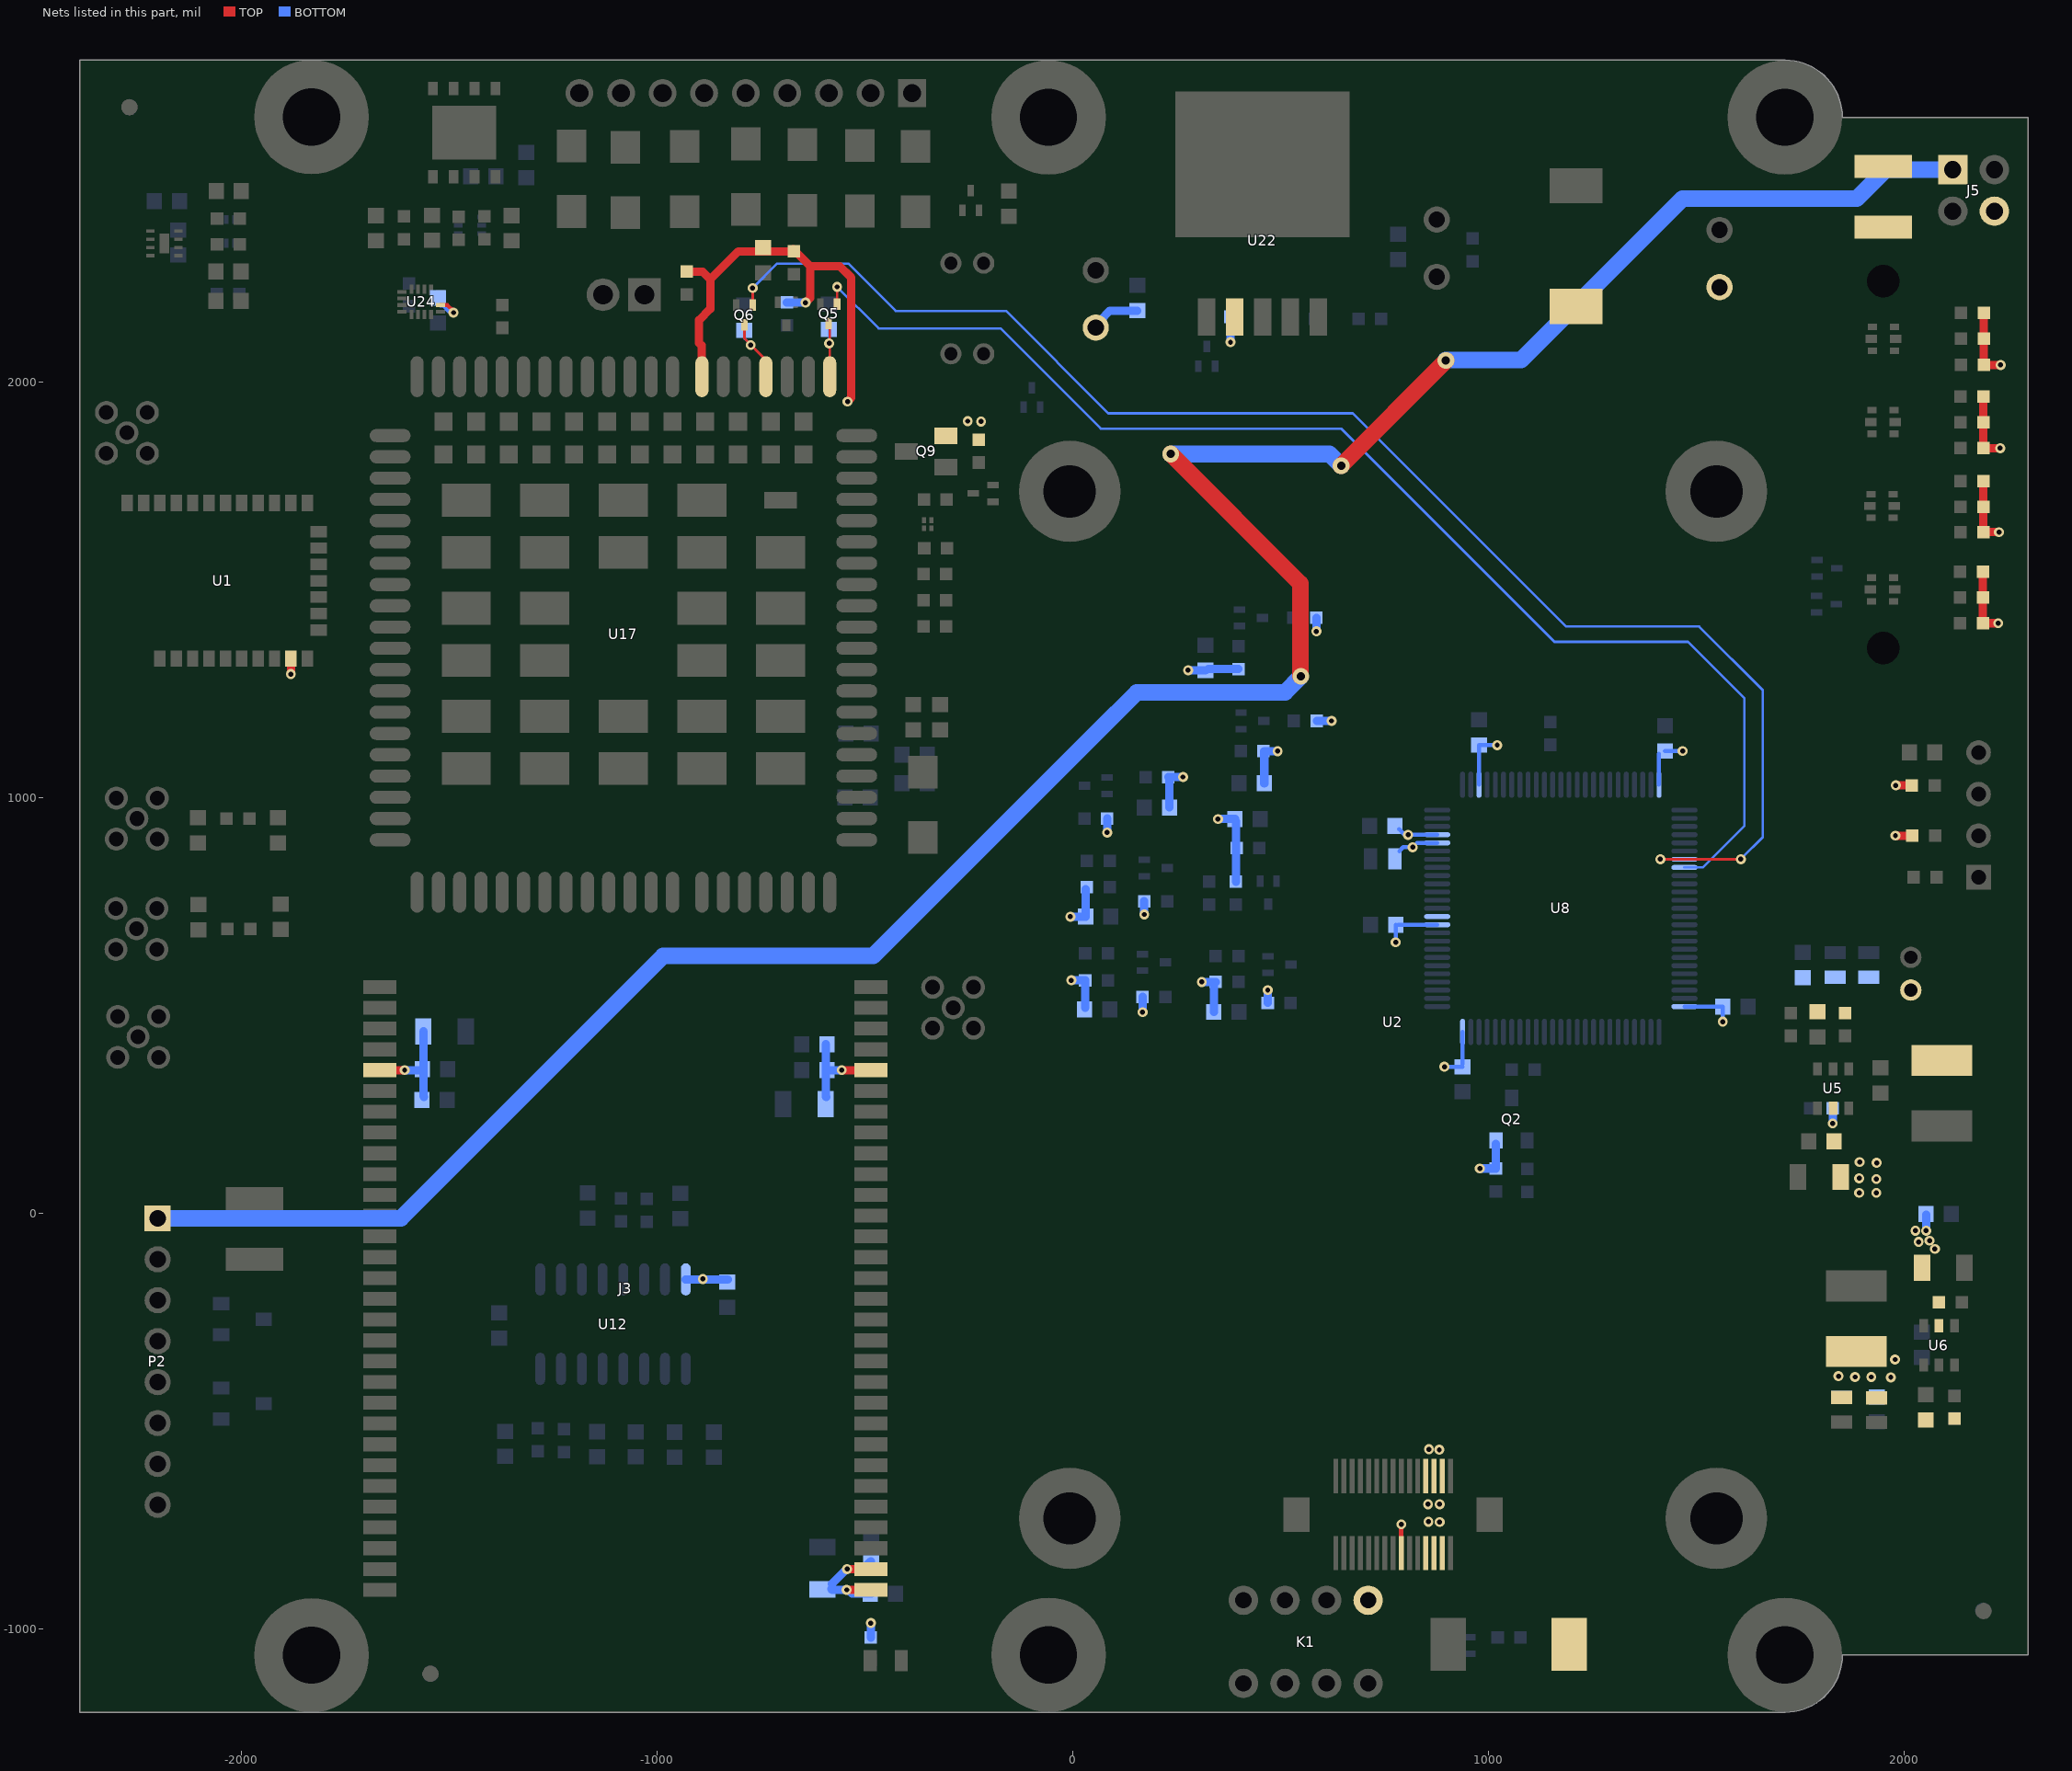
[diagram p0: the nets of this part, all layers, seen from the top]
# Altium PCB MISC84456.PcbDoc (part 5 of 5)
Units mil, origin at the board's own origin, x right, y up, seen from the top; angles counter-clockwise.
Board outline 4685.04 x 3973.82 mil, 4 copper layers (TOP, GND, POWER, BOTTOM), stack 38.4 mil thick; 219 components, 175 nets, 938 pads, 792 vias.

## Via types
v1: diameter 24, hole 12, TOP to BOTTOM, 400 vias
v2: diameter 24, hole 12, TOP to BOTTOM, tented both sides, 388 vias
v3: diameter 40, hole 20, TOP to BOTTOM, 4 vias

## Nets (pads, with @x,y where several pads share a name; then routed paths per layer and width w, separated by ;. In a path a pad name is that pad's centre, name@x,y a point inside that pad or via, vN(x,y) a via of type N, cw(c..) or ccw(c..) an arc to the next point about the centre after c; other vN are vias at no path point) (continued)
VDD_3V3: C2.1 C3.1 C11.1 C20.2 C21.2 C22.2 C38.2 C39.1 C40.1 C41.1 C42.1 C43.1 C53.1 C54.1 C55.2 C56.1 C88.1 J3.31 J3.32 J5.4 L4.2 Q2.2 R1.1 R2.1 R3.1 R17.2 R18.1 R25.2 R35.2 R38.2 R46.2 R49.2 R53.2 R55.2 R75.1 R76.1 R81.1 R82.1 R85.1 R86.1 R91.1 R92.1 R94.1 U1.9 U2.18 U2.23 U2.24 U2.25 U2.26 U2.27 U2.28 U8.11 U8.21 U8.22 U8.28 U8.50 U8.75 U8.100 U12.16 U24.14 | length 2443
  TOP w9: U24.14@-1520.59,2185.13 -1504.13,2185.13 v2@-1491,2172 ; v2@-1491.91,2171.09 -1488.81,2168 v2@-1486,2168
  TOP w11: U2.18@789.69,-816.52 v1(789.69,-747.31)
  TOP w20: v1(-1880.61,1297.61) U1.9@-1880.61,1334.99 ; v2(-544,-905) J3.31@-485.45,-905 ; v2(-543,-855) J3.32@-485.45,-855 ; v1(1978,909) R25.2@2018.5,909 ; v1(1979,1030) R35.2@2017.5,1030 ; R1.1@2188.5,1420 v1(2225,1420) ; R1.1@2188.5,1424.5 R2.1@2188.5,1482 R3.1@2188.5,1544 ; R85.1@2189.5,1639 v2(2227,1639) ; R85.1@2189.5,1645.5 R91.1@2189.5,1700 R94.1@2189.5,1762 ; R82.1@2189.5,1841 v2(2230,1841) ; R82.1@2189.5,1845.5 R86.1@2189.5,1903 R92.1@2189.5,1965 ; R75.1@2190.5,2040.5 R75.1@2190.5,2041 ; R81.1@2190.5,2166 R76.1@2190.5,2104 R75.1@2190.5,2041 ; v2(2231,2041) R75.1@2190.5,2041
  BOTTOM w10: C38.2@-1521,2184.5 -1514.5,2184.5 -1500,2170 v2@-1495,2170 ; v2@-1495,2169 -1489,2169 -1491,2167 v2(-1489.71,2167) ; v1(776.32,652.69) C54.1@776.32,695 ; C54.1@782.25,694.75 U8.11@876.11,694.75 ; C56.1@784,925 797.71,911.29 v1@806,911.29 ; C55.2@785,872 794.5,881.5 v1@817.5,881.5 ; v1(806,911) v1@806,911.29 ; v1(817,881) v1@817.5,881.5 ; U8.21@876,891 827,891 v1@817.5,881.5 ; U8.21@876,891.6 U8.21@876.11,891.6 ; U8.22@876.11,911.29 v1@806,911.29 ; v1(893.32,353.32) C11.1@937,353.32 ; C11.1@937.13,359.87 U8.100@937.13,436.88 ; U8.28@976.5,1031.36 C2.1@976.5,1124.5 ; C2.1@977,1126.69 v1(1020.32,1126.69) ; U8.50@1409.57,1031.36 C3.1@1409.57,1105.43 ; C3.1@1424,1112.69 v1(1466.32,1112.69) ; U8.75@1470.59,497.9 C53.1@1561.1,497.9 ; v1(1562.69,461.69) C53.1@1562.69,498
  BOTTOM w20: v2(-1489.71,2167) v2@-1489.6,2167 ; U12.16@-931,-158.2 v2@-891,-158.2 ; v2(-890,-157.2) v2@-891,-158.2 ; C88.1@-830.2,-158.2 v2@-891,-158.2 ; C22.2@-581,-903 -579,-905 -540,-905 -531,-914 C21.2@-484.5,-914 ; C22.2@-580,-891 -544,-855 v2(-543,-855) -505,-855 C20.2@-486,-836 ; R18.1@-486,-1019.5 v2(-486,-985) ; v1(167.5,484.5) R55.2@167.5,521 ; v1(171.5,719.5) R46.2@171.5,751 ; R53.2@468.5,507 v1(468.5,537.5) ; R49.2@586.5,1185 v1(622,1185) ; v1(978.5,108.5) R38.2@1017,108.5 Q2.2@1017,168
  other v1: 882,-742 855,-741 854,-699 882,-699 881,-568 856,-567 1967,-394 1881,-393 1920,-393 1841,-391 1977,-351
VDD_5V: C5.2 C6.1 C7.1 C8.2 C9.2 C10.2 C25.1 C26.1 C27.1 C28.1 C29.1 C91.1 C101.1 J3.5 J3.56 L3.2 Q9.2 R11.2 R29.1 R65.2 U22.2 | length 652.7
  TOP w20: J3.5@-1666.55,345 v2(-1607,345) ; v2(-556,345) J3.56@-485.45,345
  BOTTOM w20: v2@-1603,345 C9.2@-1562.5,345 ; C10.2@-1562.16,438 -1562.16,282.16 C8.2@-1561,281 ; C7.1@-594.5,407 -594.5,281.5 C5.2@-593,280 ; C6.1@-592,345 v2(-556,345) ; C91.1@65,2148 88.69,2171.69 C101.1@155,2171.69 ; R65.2@378.5,2157 378.5,2099.5 379,2099 v2(379,2096)
  other v2: -221,1905 -253,1906
VDD_12V: C4.1 C30.2 C31.2 C44.2 C46.2 D1.2 D3.2 K1.1 R10.1 R12.2 R19.2 U5.5 U6.5 | length 68.5
  BOTTOM w20: v1@1827.5,222.5 R12.2@1827.5,253 ; v2(2052,-41) C46.2@2052,-3
  other v1: 1827,217
  other v2: 2073,-85 2034,-68 2060,-65 2026,-41 1891,50 1932,50 1932,83 1891,85 1933,122 1892,124
VDD_EXT: C57.1 C58.2 C59.1 C60.1 C61.2 C62.2 C63.2 C64.2 R30.1 R31.1 R39.2 R40.2 R41.1 R43.2 R44.1 R45.1 R48.1 R51.1 R54.1 R56.1 R77.1 U17.7 | length 1990.2
  TOP w20: R77.1@-922,2265 -890,2265 -872,2247 ; U17.7@-893,2046 -893,2088 -899,2094 -899,2149 -872,2176 -872,2247 ; R31.1@-672.5,2319.5 -632,2279 ; R31.1@-671,2314.5 -804.5,2314.5 -872,2247 ; v2(-643,2191) -632,2202 -632,2279 ; v2(-542,1953) -533,1962 -533,2251 -561,2279 -632,2279
  BOTTOM w20: R30.1@-688,2191.5 v2@-643.5,2191.5 ; v1(-6,714) C61.2@30.69,714 R48.1@30.69,780.69 ; v1(-4,561) R56.1@29.5,561 C64.2@29.5,495.5 ; v1(82.5,916.5) R45.1@82.5,950 ; R43.2@229.5,1050 v1(265,1050) ; C60.1@232.32,977 R43.2@232.32,1048.69 ; v1(277,1307) C59.1@318.69,1307 ; v1(310,557) R54.1@343.5,557 ; C59.1@325.5,1309.5 R40.2@398,1309.5 ; C63.2@338.69,485 R54.1@338.69,549.69 ; v1(349,949) C57.1@389.69,949 ; R41.1@392,798.5 C57.1@392,943 ; C62.2@460.32,1035 460.32,1112.32 v1(492.32,1112.32) ; v1(585.5,1400.5) R44.1@585.5,1433
VDD_IN: J5.1 P2.1 R10.2 | length 6252
  TOP w40: v3(235,1827) 547,1515 v3@547,1293 ; v3(645,1799) v3@898,2052
  BOTTOM w40: P2.1@-2201,-11.51 -1616.51,-11.51 -985,620 -480,620 24,1124 ; 104,1204 24,1124 ; v3(235,1827) 617,1827 v3(645,1799) ; v3@547,1291 510,1254 154,1254 24,1124 ; v3@897,2053 1078,2053 1466,2441 1885,2441 1955,2511 J5.1@2116,2511
  other v3: 548,1292 897,2052
W_DISABLE_MCU: Q6.1 U8.57 | length 3759.8
  TOP w6: Q6.1@-770.12,2184.87 v2(-770.12,2226.12) ; v1(1412.77,852.23) v1(1606.23,852.23)
  BOTTOM w6: v2(-770.12,2226.12) -711.25,2285 -540,2285 -426,2171 -366,2171 ; -202,2171 -366,2171 ; v1(1412.77,852.23) U8.57@1470.59,852.23 ; v1@1609,855 1659,905 1659,1259 1506,1412 1186,1412 673,1925 85,1925 -161,2171 -366,2171
W_DISABLE_MODULE: C48.1 Q6.3 U17.4 | length 207
  TOP w6: Q6.3@-790,2141 -790,2105 -738.48,2053.48 U17.4@-738.48,2013.08
  BOTTOM w6: C48.1@-790,2120 C48.1@-790,2124.69 C48.1@-790,2135 ; C48.1@-789,2120 -789,2103.66 v2@-770.34,2085
  other v2: -775,2089
WAKEUP_IN_MCU: Q5.1 U8.58 | length 3247.2
  TOP w6: Q5.1@-567.12,2187.87 v2(-567.12,2228.88)
  BOTTOM w6: v2(-567.12,2228.88) -467.25,2129 -324,2129 ; -202,2129 -324,2129 ; U8.58@1470.59,832.55 1514.55,832.55 1615,933 1615,1239 1479,1375 1158,1375 645,1888 67,1888 -174,2129 -324,2129
WAKEUP_IN_MODULE: C47.1 Q5.3 U17.1 | length 169.4
  TOP w6: U17.1@-584.94,2013.08 -584.94,2136.06 Q5.3@-584,2137
  BOTTOM w6: C47.1@-587,2137.69 -586,2136.69 v2(-586,2093)
XTAL1: U8.12
pads on no net: J3.7 J3.8 J3.10 J3.11 J3.12 J3.13 J3.15 J3.16 J3.17 J3.19 J3.20 J3.21 J3.22 J3.23 J3.24 J3.26 J3.27 J3.28 J3.29 J3.30 J3.41 J3.42 J3.44 J3.45 J3.46 J3.48 J3.49 J3.50 J3.51 J3.53 J3.54 U1.2 U1.3 U1.4 U1.5 U1.6 U1.8 U1.11 U1.12 U1.13 U1.14 U1.15 U1.19 U1.20 U1.21 U1.22 U1.27 U2.0 U2.2 U2.4 U2.6 U2.8 U2.10 U2.15 U2.16 U2.17 U2.29 U2.31 U8.1 U8.2 U8.3 U8.4 U8.5 U8.6 U8.7 U8.8 U8.9 U8.13 U8.18 U8.24 U8.29 U8.30 U8.31 U8.32 U8.33 U8.34 U8.35 U8.36 U8.54 U8.63 U8.64 U8.65 U8.66 U8.67 U8.73 U8.77 U8.81 U8.82 U8.84 U8.85 U8.86 U8.87 U8.88 U8.89 U8.90 U8.91 U8.92 U8.93 U8.97 U8.98 U17.3 U17.18 U17.23 U17.24 U17.25 U17.26 U17.27 U17.28 U17.29 U17.30 U17.31 U17.32 U17.33 U17.34 U17.37 U17.38 U17.39 U17.40 U17.41 U17.42 U17.43 U17.44 U17.45 U17.55 U17.113 U17.114 U17.116 U17.117 U17.118 U17.119 U17.120 U17.121 U17.122 U17.123 U17.124 U17.125 U17.126 U17.127 U17.128 U17.129 U17.130 U17.131 U17.132 U17.133 U17.134 U17.135 U17.136 U17.137 U17.138 U17.139 U17.140 U17.141 U17.142 U17.143 U17.144 U20.2 U20.4 U20.5 U23.4 U25.2 U25.4 U25.5 U26.6
copper on no net: | length 375.1
  BOTTOM w20: -1706,913 -1527,734 v2(-1527,612)

## Polygon pours and split planes (outlines as drawn)
VBAT on TOP "BottomLayer-No Net" (solid, remove dead copper): 498,2162 498,2123 498,2060 512,2046 532,2026 568,2026 678,2026 749,2097 756,2104 815,2104 913,2104 923,2114 947,2138 947,2154 947,2274 940,2281 916,2305 795,2305 734,2244 665,2175 665,2134 665,2123 652,2110 637,2095 615,2095 564,2095 555,2104 547,2112 547,2121 547,2200 543,2204 542,2205 533,2205 506,2205 500,2199 498,2197 498,2162
VDD_12V on TOP "BottomLayer-No Net" (solid, remove dead copper): 1108,1787 1108,1821 1108,2209 1155,2256 1174,2275 1524,2275 1607,2275 1653,2321 1746,2414 1892,2414 2023,2414 2038,2399 2041,2396 2041,2379 2041,2331 2036,2326 2023,2313 1988,2313 1888,2313 1843,2268 1630,2055 1566,2055 1489,2055 1439,2005 1347,1913 1347,1805 1347,1793 1331,1777 1324,1770 1314,1770 1125,1770 1108,1787
VBAT on TOP "BottomLayer-No Net" (solid, remove dead copper): -344,2275 -344,2068 -326,2050 -317,2041 -301,2041 -280,2041 -273,2048 -265,2056 -265,2274 -265,2309 -280,2324 -282,2326 -302,2326 -315,2326 -330,2311 -344,2297 -344,2275
VDD_12V on TOP "BottomLayer-No Net" (solid, remove dead copper): 672,-924 672,-964 686,-978 700,-992 741,-992 792,-992 833,-951 841,-943 862,-943 958,-943 982,-967 982,-1011 982,-1120 998,-1136 1021,-1159 1050,-1159 1269,-1159 1298,-1130 1362,-1066 1362,-903 1362,-644 1455,-551 1657,-349 1657,-183 1657,-161 1699,-119 1723,-95 1877,-95 1983,-95 2000,-112 2009,-121 2009,-151 2009,-166 2025,-182 2027,-184 2035,-184 2044,-184 2058,-198 2067,-207 2067,-276 2067,-281 2070,-284 2074,-288 2080,-288 2092,-288 2096,-284 2098,-282 2098,9 2098,56 2060,94 2056,98 2033,98 1992,98 1897,193 1893,197 1874,197 1859,197 1844,212 1841,215 1841,250 1841,268 1837,272 1831,272 1820,272 1817,269 1815,267 1815,264 1815,208 1810,203 1808,201 1808,189 1808,26 1802,20 1798,16 1720,16 1670,16 1645,41 1527,159 1527,472 1527,662 1478,711 1466,723 1406,723 1348,723 1326,745 1203,868 1203,1175 1203,1228 1308,1333 1347,1372 1347,1570 1347,1806 1302,1851 1300,1853 1242,1853 1175,1853 1108,1786 1108,1188 1108,782 1214,676 1265,625 1302,625 1346,625 1360,611 1376,595 1376,560 1376,512 1343,479 1226,362 1226,-116 1226,-182 1183,-225 1140,-268 1140,-619 1140,-979 1123,-996 1073,-996 1069,-996 1037,-964 963,-890 715,-890 693,-890 673,-910 672,-911 672,-925
VDD_5V on TOP "BottomLayer-No Net" (solid, remove dead copper): 1767,508 1767,470 1771,466 1787,466 1889,466 1903,452 1985,370 1985,352 1985,335 1990,330 1999,321 2016,321 2161,321 2166,326 2181,341 2181,363 2181,488 2156,513 2105,564 2015,564 1975,564 1953,542 1926,515 1836,515 1774,515 1767,508
GND_IN on TOP "BottomLayer-No Net" (solid, remove dead copper): -2241,-105 -2241,-135 -2234,-142 -2224,-152 -2186,-152 -1881,-152 -1869,-140 -1865,-136 -1865,-114 -1865,-88 -1875,-78 -1882,-71 -1920,-71 -2224,-71 -2233,-80 -2241,-88 -2241,-105
VDD_3V3 on TOP "BottomLayer-No Net" (solid, remove dead copper): 842,-596 842,-857 845,-860 853,-860 892,-860 894,-858 895,-857 895,-848 895,-557 890,-552 887,-549 877,-549 853,-549 850,-552 842,-560 842,-594
VDD_5V on TOP "BottomLayer-No Net" (solid, remove dead copper): 8,2130 8,2068 18,2058 47,2029 281,2029 383,2029 399,2045 413,2059 413,2116 413,2203 411,2205 409,2207 402,2207 371,2207 369,2205 364,2200 364,2185 364,2096 356,2088 317,2088 249,2088 221,2116 165,2172 82,2172 38,2172 18,2152 8,2142 8,2130
NetD1_1 on TOP "BottomLayer-No Net" (solid, remove dead copper): 674,-1115 674,-1141 674,-1159 680,-1165 684,-1169 702,-1169 913,-1169 945,-1137 959,-1123 959,-1095 959,-978 950,-969 944,-963 924,-963 867,-963 850,-980 764,-1066 726,-1066 704,-1066 689,-1081 674,-1096 674,-1115
NetC33_1 on TOP "BottomLayer-No Net" (solid, remove dead copper, pour order 1006): 1800,-161 1800,-211 1806,-217 1817,-228 1835,-228 1930,-228 1973,-271 1992,-290 2032,-290 2050,-290 2056,-284 2058,-282 2058,-274 2058,-222 2046,-210 2037,-201 2020,-201 2010,-201 2000,-191 1991,-182 1991,-155 1991,-143 1981,-133 1973,-125 1960,-125 1818,-125 1807,-136 1800,-143 1800,-160
VDD_3V3 on TOP "BottomLayer-No Net" (solid, remove dead copper, pour order 1007): 1793,-336 1793,-444 1809,-460 1837,-460 1970,-460 1977,-467 1989,-479 1989,-495 1989,-505 1995,-511 2001,-517 2038,-517 2132,-517 2136,-513 2139,-510 2139,-505 2139,-484 2136,-481 2134,-479 2129,-479 2025,-479 2016,-470 1994,-448 1994,-421 1994,-322 1971,-299 1964,-292 1950,-292 1815,-292 1807,-300 1793,-314 1793,-335
VDD_12V on TOP "BottomLayer-No Net" (solid, remove dead copper, pour order 1008): 2012,-101 2012,-169 2022,-179 2028,-185 2036,-185 2044,-185 2052,-193 2067,-208 2067,-244 2067,-281 2073,-287 2074,-288 2079,-288 2094,-288 2095,-287 2098,-284 2098,-277 2098,-68 2089,-59 2084,-54 2066,-54 2025,-54 2019,-60 2012,-67 2012,-101
NetC23_1 on TOP "BottomLayer-No Net" (solid, remove dead copper, pour order 1009): 1853,260 1853,228 1869,212 1871,210 1895,210 1898,210 1906,210 1982,134 1991,125 2064,125 2144,125 2167,148 2182,163 2182,186 2182,236 2170,248 2166,252 2149,252 2030,252 1995,287 1973,309 1957,309 1929,309 1920,300 1896,276 1873,276 1862,276 1857,271 1853,267 1853,260
VDD_IN on TOP "BottomLayer-No Net" (solid, remove dead copper, pour order 1015): 1863,2553 1863,2508 1873,2498 1902,2469 2078,2469 2148,2469 2158,2479 2163,2484 2163,2513 2163,2561 2147,2577 2132,2592 2035,2592 1882,2592 1870,2580 1863,2573 1863,2552
VDD_5V on TOP "BottomLayer-No Net" (solid, remove dead copper, pour order 1019): -337,1899 -337,1870 -337,1854 -333,1850 -330,1847 -312,1847 -212,1847 -205,1854 -199,1860 -199,1875 -199,1915 -201,1917 -205,1921 -209,1921 -322,1921 -332,1911 -337,1906 -337,1899
GND on TOP "BottomLayer-No Net" (solid, remove dead copper, pour order 1023): -2672.84,2567.76 -2672.84,-1287.24 -2535.84,-1424.24 -2383.84,-1576.24 -1544.84,-1576.24 2077.16,-1576.24 2302.16,-1351.24 2541.16,-1112.24 2541.16,-411.24 2541.16,2704.76 2403.16,2842.76 2100.16,3145.76 1290.16,3145.76 -2303.84,3145.76 -2549.84,2899.76 -2665.84,2783.76 -2665.84,2581.76
VBAT on TOP "BottomLayer-No Net" (solid, remove dead copper, pour order 1000): -418,1103 -418,1084 -418,1046 -407,1035 -391,1019 -367,1019 -293,1019 -253,1059 -204,1108 -204,1131 -204,1170 -213,1179 -217,1183 -223,1183 -399,1183 -405,1177 -418,1164 -418,1104
GND on BOTTOM "BottomLayer-No Net" (solid, remove dead copper): -2907.62,2704 -2907.62,-1226 -2714.62,-1419 -2439.62,-1694 -1689.62,-1694 1735.38,-1694 2047.38,-1382 2422.38,-1007 2422.38,-407 2422.38,2729 2109.38,3042 1909.38,3242 -1289.62,3242 -2368.62,3242 -2907.62,2703
VDD_5V on BOTTOM "BottomLayer-No Net" (solid, remove dead copper): 1732,573 1732,563 1732,551 1738,545 1787,496 1990,496 2031,496 2045,510 2051,516 2051,532 2051,551 2042,560 2038,564 2028,564 1982,564 1969,577 1960,586 1939,586 1739,586 1736,583 1732,579 1732,573
VDD_3V3 on BOTTOM "BottomLayer-No Net" (solid, remove dead copper, pour order 1027): 1799,-389 1799,-434 1811,-446 1824,-459 1841,-459 1958,-459 1967,-450 1991,-426 1991,-384 1991,-335 1982,-326 1978,-322 1971,-322 1955,-322 1945,-332 1914,-363 1853,-363 1818,-363 1804,-377 1799,-382 1799,-388
GND on GND (split plane): 1721.84,2753.94 1731.03,2752.85 1740.1,2751.05 1749,2748.54 1757.67,2745.34 1766.07,2741.46 1774.14,2736.95 1781.83,2731.81 1789.1,2726.08 1795.89,2719.8 1802.16,2713.01 1807.89,2705.75 1813.03,2698.06 1817.55,2689.99 1821.42,2681.59 1824.62,2672.91 1827.13,2664.01 1828.94,2654.94 1830.02,2645.76 1830.36,2637.15 1830.3,2636.52 1830.68,2632.6 1831.83,2628.83 1833.68,2625.35 1836.18,2622.31 1839.23,2619.81 1842.7,2617.95 1846.47,2616.81 1850.39,2616.42 2276.78,2616.42 2276.78,-1041.62 1850.39,-1041.62 1846.47,-1042 1842.7,-1043.15 1839.23,-1045 1836.18,-1047.5 1833.68,-1050.55 1831.83,-1054.02 1830.68,-1057.79 1830.3,-1061.71 1830.36,-1062.35 1830.02,-1070.95 1828.94,-1080.14 1827.13,-1089.21 1824.62,-1098.11 1821.42,-1106.79 1817.55,-1115.19 1813.03,-1123.26 1807.89,-1130.95 1802.16,-1138.21 1795.89,-1145 1789.1,-1151.28 1781.83,-1157 1774.14,-1162.14 1766.07,-1166.66 1757.67,-1170.53 1749,-1173.73 1740.1,-1176.24 1731.03,-1178.05 1721.84,-1179.14 1713.24,-1179.47 1712.6,-1179.41 -2368.07,-1179.41 -2368.07,2754.21 1712.6,2754.21 1713.24,2754.28
VDD_3V3 on POWER (split plane): -1125.09,901 -1124.74,898.39 -1123.73,895.96 -1122.13,893.87 -1056.13,827.87 -1054.04,826.26 -1051.61,825.26 -1049,824.91 -184.09,824.91 -184.09,699 -183.74,696.39 -182.73,693.96 -181.13,691.87 -14.13,524.87 -12.04,523.26 -9.61,522.26 -7,521.91 29,521.91 31.61,522.26 34.04,523.26 36.13,524.87 75.13,563.87 76.74,565.96 77.45,567.68 77.74,568.39 78.09,571 78.09,702.82 127.18,751.91 224.82,751.91 256.91,719.82 256.91,551 257.26,548.39 258.27,545.96 259.87,543.87 294.87,508.87 296.96,507.26 299.39,506.26 302,505.91 352,505.91 354.61,506.26 357.04,507.26 359.13,508.87 425.13,574.87 426.74,576.96 427.74,579.39 428.09,582 428.09,875.82 550.13,997.87 551.74,999.96 552.74,1002.39 553.09,1005 553.09,1258.82 661,1366.74 737.87,1289.87 739.96,1288.26 742.39,1287.26 745,1286.91 1330.82,1286.91 1486.91,1130.82 1486.91,599 1487.26,596.39 1488.27,593.96 1489.87,591.87 1584.91,496.82 1584.91,279.18 1318.82,13.09 -179.82,13.09 -556.87,390.13 -558.96,391.74 -561.39,392.74 -564,393.09 -1664,393.09 -1666.61,392.74 -1668.33,392.03 -1669.04,391.74 -1671.13,390.13 -1698.13,363.13 -1699.73,361.04 -1700.74,358.61 -1701.09,356 -1701.09,157 -1700.74,154.39 -1699.73,151.96 -1698.13,149.87 -1587.13,38.87 -1585.04,37.26 -1582.61,36.26 -1580,35.91 -700.18,35.91 -339.13,-325.13 -337.04,-326.74 -335.32,-327.45 -334.61,-327.74 -332,-328.09 1567,-328.09 1569.61,-327.74 1572.04,-326.74 1574.13,-325.13 2054.13,154.87 2055.74,156.96 2056.74,159.39 2057.09,162 2057.09,626 2056.74,628.61 2055.74,631.04 2054.13,633.13 2053.57,633.57 2053.13,634.13 1859.09,828.18 1859.09,2616.42 2276.78,2616.42 2276.78,-1041.62 1850.39,-1041.62 1846.47,-1042 1842.7,-1043.15 1839.23,-1045 1836.18,-1047.5 1833.68,-1050.55 1831.83,-1054.02 1830.68,-1057.79 1830.3,-1061.71 1830.36,-1062.35 1830.02,-1070.95 1828.94,-1080.14 1827.13,-1089.21 1824.62,-1098.11 1821.42,-1106.79 1817.55,-1115.19 1813.03,-1123.26 1807.89,-1130.95 1802.16,-1138.21 1795.89,-1145 1789.1,-1151.28 1781.83,-1157 1774.14,-1162.14 1766.07,-1166.66 1757.67,-1170.53 1749,-1173.73 1740.1,-1176.24 1731.03,-1178.05 1721.84,-1179.14 1713.24,-1179.47 1712.6,-1179.41 -2368.07,-1179.41 -2368.07,2754.21 -1125.09,2754.21
VDD_5V on POWER (split plane): 1721.84,2753.94 1731.03,2752.85 1740.1,2751.05 1749,2748.54 1757.67,2745.34 1766.07,2741.46 1774.14,2736.95 1781.83,2731.81 1789.1,2726.08 1795.89,2719.8 1802.16,2713.01 1807.89,2705.75 1813.03,2698.06 1817.55,2689.99 1821.42,2681.59 1824.62,2672.91 1827.13,2664.01 1828.94,2654.94 1830.02,2645.76 1830.36,2637.15 1830.3,2636.52 1830.68,2632.6 1831.83,2628.83 1833.68,2625.35 1836.18,2622.31 1838.91,2620.07 1838.91,2620 1838.91,1804 1838.91,824 1839.26,821.39 1840.27,818.96 1841.87,816.87 2036.91,621.82 2036.91,166.18 1562.82,-307.91 -327.82,-307.91 -688.87,53.13 -690.96,54.74 -693.39,55.74 -696,56.09 -1575.82,56.09 -1680.91,161.18 -1680.91,351.82 -1659.82,372.91 -568.18,372.91 -191.13,-4.13 -189.04,-5.74 -188.33,-6.03 -186.61,-6.74 -184,-7.09 1323,-7.09 1325.61,-6.74 1328.04,-5.74 1330.13,-4.13 1602.13,267.87 1603.74,269.96 1604.24,271.17 1604.74,272.39 1605.09,275 1605.09,501 1604.74,503.61 1604.45,504.32 1603.74,506.04 1602.13,508.13 1507.09,603.18 1507.09,1135 1506.74,1137.61 1505.74,1140.04 1504.13,1142.13 1342.13,1304.13 1340.04,1305.74 1337.61,1306.74 1335,1307.09 749.18,1307.09 669.09,1387.18 669.09,1542 668.74,1544.61 667.74,1547.04 666.13,1549.13 609.76,1605.51 609.74,1605.61 608.74,1608.04 607.13,1610.13 605.04,1611.74 602.61,1612.74 600,1613.09 599,1613.09 596.39,1612.74 594.81,1612.09 -147.82,1612.09 -322.91,1787.18 -322.91,1963.87 -321.96,1964.26 -319.87,1965.87 -281.82,2003.91 -193,2003.91 -190.39,2004.26 -187.96,2005.26 -185.87,2006.87 -6.82,2185.91 214.82,2185.91 329.87,2070.87 331.96,2069.26 334.39,2068.26 337,2067.91 818,2067.91 820.61,2068.26 823.04,2069.26 825.13,2070.87 961.13,2206.87 962.74,2208.96 963.74,2211.39 964.09,2214 964.09,2754.21 1712.6,2754.21 1713.24,2754.28
VBAT on POWER (split plane): 943.91,2218.18 813.82,2088.09 341.18,2088.09 226.13,2203.13 224.04,2204.74 221.61,2205.74 219,2206.09 -11,2206.09 -13.61,2205.74 -16.04,2204.74 -18.13,2203.13 -197.18,2024.09 -286,2024.09 -288.61,2023.74 -290.33,2023.03 -291.04,2022.74 -293.13,2021.13 -331,1983.26 -374.87,2027.13 -376.96,2028.74 -379.39,2029.74 -382,2030.09 -534,2030.09 -536.61,2029.74 -539.04,2028.74 -541.13,2027.13 -575.13,1993.13 -576.73,1991.04 -577.74,1988.61 -578.09,1986 -578.09,1963 -578.09,1960 -578.09,1425 -577.74,1422.39 -576.73,1419.96 -575.13,1417.87 -455.13,1297.87 -453.04,1296.26 -450.61,1295.26 -448,1294.91 -273.18,1294.91 -184.09,1205.82 -184.09,845.09 -1044.82,845.09 -1104.91,905.18 -1104.91,2754.21 943.91,2754.21
VDD_EXT on POWER (split plane): -343.09,1966.82 -343.09,1783 -342.74,1780.39 -341.73,1777.96 -340.13,1775.87 -159.13,1594.87 -157.04,1593.26 -154.61,1592.26 -152,1591.91 594.82,1591.91 648.91,1537.82 648.91,1390.89 648.27,1390.04 647.26,1387.61 646.91,1385 647.26,1382.39 647.51,1381.78 535.87,1270.13 534.27,1268.04 533.26,1265.61 532.91,1263 532.91,1009.18 410.87,887.13 409.27,885.04 408.26,882.61 407.91,880 407.91,586.18 347.82,526.09 306.18,526.09 277.09,555.18 277.09,724 276.74,726.61 276.45,727.32 275.74,729.04 274.13,731.13 236.13,769.13 234.04,770.74 231.61,771.74 229,772.09 123,772.09 120.39,771.74 119.68,771.45 117.96,770.74 115.87,769.13 60.87,714.13 59.27,712.04 58.26,709.61 57.91,707 57.91,575.18 24.82,542.09 -2.82,542.09 -163.91,703.18 -163.91,1210 -164.26,1212.61 -164.76,1213.83 -165.26,1215.04 -166.87,1217.13 -261.87,1312.13 -263.96,1313.74 -266.39,1314.74 -269,1315.09 -443.82,1315.09 -557.91,1429.18 -557.91,1963 -557.91,1981.82 -529.82,2009.91 -386.18,2009.91

## Keep-outs
Keep-Out Layer:
  the board outline again, w5

## Other copper
TOP:
  pour cut-out: -1629,-974 -530,-974 -530,603 -1629,603
  pour cut-out: -1593,854 -1562,823 -602,823 -572,853 -572,1935 -599,1962 -1562,1962 -1593,1931
POWER (plane layer: these items are gaps in the copper):
  lines w20: -1115,2773 -1115,901 -1049,835 -181,835 ; -568,1960 -568,1986 -534,2020 -382,2020 -333,1971 -333,1783 -152,1602 599,1602 659,1542 659,1379 543,1263 543,1005 418,880 418,582 352,516 302,516 267,551 267,724 229,762 123,762 68,707 68,571 29,532 -7,532 -174,699 -174,1210 -269,1305 -448,1305 -568,1425 -568,1963 ; -327,1973 -286,2014 -193,2014 -11,2196 219,2196 337,2078 818,2078 954,2214 954,2766 ; 599,1603 600,1603 ; 657,1385 745,1297 1335,1297 1497,1135 1497,599 1595,501 1595,275 1323,3 -184,3 -564,383 -1664,383 -1691,356 -1691,157 -1580,46 -696,46 -332,-318 1567,-318 2047,162 2047,626 ; 1849,1804 1849,2632 ; 1849,2620 1849,824 2046,627

## Silkscreen, mask and mechanical layers (free items; w line width, h text height)
Top Overlay:
  text "GND" at 2189,2313 h40
  text "VDD" at 2075,2312 h40
  text "ACIN" at 2073,2269 h40
  text "3.3V" at 2193,2269 h40
  text "Agr-Ctrl_3G_V1.0  2021-5-28" at 228,1169 h50
  text "RST" at 2281,1085 h40 r90
  text "GND" at 2280,974 h40 r90
  text "JTMS" at 2279,858 h40 r90
  text "JTCK" at 2278,752 h40 r90
  text "VDD" at -2066,-7 h40 r90
  text "GND_IN" at -2067,-182 h40 r90
  text "TX_G" at -2084,-239 h40
  text "RX_G" at -2074,-321 h40
  text "TX_D" at -2078,-423 h40
  text "RX_D" at -2082,-515 h40
  text "GND" at -2079,-623 h40
  text "BOOT" at -2082,-716 h40
Bottom Overlay:
  text "TX" at -1098,2601 h40 r270
  text "DP" at -899,2601 h40 r270
  text "RX" at -1005,2600 h40 r270
  text "DM" at -798,2596 h40 r270
  text "GND" at -501,2567 h40 r270
  text "VBAT" at -397,2548 h40 r270
  text "VBUS" at -703,2547 h40 r270
  text "TX_FC20" at -1191,2498 h40 r270
  text "PWRKEY" at -598,2493 h40 r270
Mechanical 2:
  circle w5: c-1830.71,-1061.71 r137.8
  circle w5: c-1830.71,-1061.71 r68.9
  circle w5: c-59.06,-1061.71 r137.8
  circle w5: c-59.06,-1061.71 r68.9
  circle w5: c1712.6,2636.52 r137.8
  circle w5: c1712.6,2636.52 r68.9
  circle w5: c-59.06,2636.52 r68.9
  circle w5: c-59.06,2636.52 r137.8
  circle w5: c-1830.71,2636.52 r137.8
  circle w5: c-1830.71,2636.52 r68.9
  circle w5: c1712.6,-1061.71 r68.9
  circle w5: c1712.6,-1061.71 r137.8
  lines w5: -1830.71,-1199.51 -1830.71,2774.31 ; 1929.12,1321.55 cw(c1929.12,1360.92) 1929.12,1400.29 1968.49,1400.29 cw(c1968.49,1360.92) 1968.49,1321.55 ; 0,0 1574.8,0 1574.8,1574.8 0,1574.8 0,0 ; 1799.54,1315.37 2294.85,1315.37 2294.85,2306.01 1799.54,2306.01 1799.54,1315.37 ; 1834.63,1471.75 1834.63,1530.8 1903.53,1530.8 1903.53,1471.75 1834.63,1471.75 ; 1834.63,1672.14 1834.63,1731.2 1903.53,1731.2 1903.53,1672.14 1834.63,1672.14 ; 1834.63,1872.54 1834.63,1931.59 1903.53,1931.59 1903.53,1872.54 1834.63,1872.54 ; 1834.63,2072.93 1834.63,2131.99 1903.53,2131.99 1903.53,2072.93 1834.63,2072.93 ; 1929.12,2203.44 cw(c1929.12,2242.81) 1929.12,2282.18 1968.49,2282.18 cw(c1968.49,2242.81) 1968.49,2203.44 1929.12,2203.44 ; 1994.08,1471.75 2062.98,1471.75 2062.98,1530.8 1994.08,1530.8 1994.08,1471.75 ; 1994.08,1672.14 1994.08,1731.2 2062.98,1731.2 2062.98,1672.14 1994.08,1672.14 ; 1994.08,1872.54 2062.98,1872.54 2062.98,1931.59 1994.08,1931.59 1994.08,1872.54 ; 1994.08,2072.93 2062.98,2072.93 2062.98,2131.99 1994.08,2131.99 1994.08,2072.93
DRAWING_ORIGIN:
  lines w1: -2516.13,-14292.86 -2466.13,-14292.86 ; -2491.13,-14317.86 -2491.13,-14267.86